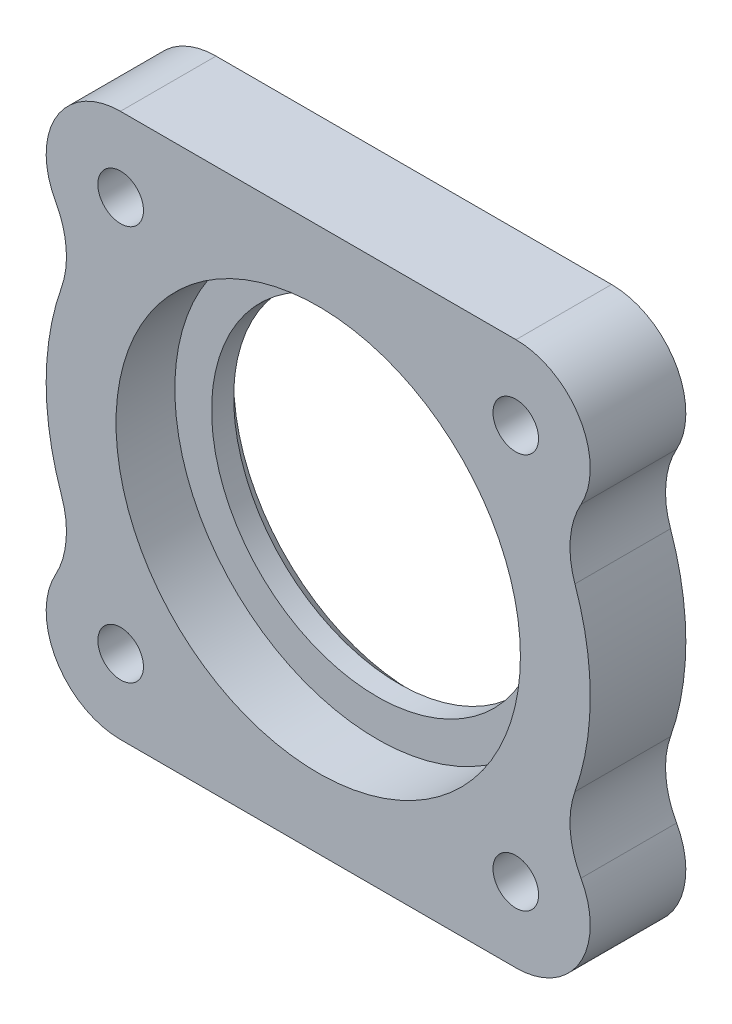
SolidWorks part; units mm, degrees
material "AL-1#"
ref_plane "前视基准面" through (0, 0, 0) normal (0, 0, 1) x (1, 0, 0)
ref_plane "上视基准面" through (0, 0, 0) normal (0, 1, 0) x (1, 0, 0)
ref_plane "右视基准面" through (0, 0, 0) normal (1, 0, 0) x (0, 0, -1)
sketch "草图1" plane through (0, 0, 0) normal (0, 0, 1) x (1, 0, 0)
  line L1 (-26.9, 37) -> (26.9, 37)
  line L5 (-37, 0) -> (-37, 44.6365) construction
  line L6 (26.9, 37) -> (26.9, 26.9) construction
  line L7 (-1000, 0) -> (49000, 0) construction
  line L10 (-26.9, 37) -> (-26.9, 26.9) construction
  line L12 (-37, 0) -> (37, 0)
  line L13 (0, -37) -> (0, 37) construction
  line L14 (-26.9, -37) -> (-26.9, -26.9) construction
  line L15 (26.9, -37) -> (26.9, -26.9) construction
  line L16 (-26.9, -37) -> (26.9, -37)
  arc A0 (-34.9172, 12.239) -> (-34.9172, -12.239) centre (0, 0) ccw
  arc A4 (-35.7394, 22.0138) -> (-26.9, 37) centre (-26.9, 26.9) cw
  arc A5 (-34.9172, 12.239) -> (-35.7394, 22.0138) centre (-46.2416, 16.2084) ccw
  arc A6 (34.9172, 12.239) -> (35.7394, 22.0138) centre (46.2416, 16.2084) cw
  arc A7 (35.7394, 22.0138) -> (26.9, 37) centre (26.9, 26.9) ccw
  arc A8 (34.9172, 12.239) -> (34.9172, -12.239) centre (0, 0) cw
  arc A9 (35.7394, -22.0138) -> (26.9, -37) centre (26.9, -26.9) cw
  arc A10 (34.9172, -12.239) -> (35.7394, -22.0138) centre (46.2416, -16.2084) ccw
  arc A11 (-34.9172, -12.239) -> (-35.7394, -22.0138) centre (-46.2416, -16.2084) cw
  arc A12 (-35.7394, -22.0138) -> (-26.9, -37) centre (-26.9, -26.9) ccw
  dimension "D2" = 10.1
  dimension "D5" = 24
extrude "凸台-拉伸1" add sketch "草图1" along normal blind 13 contours A11 A12 L16 A9 A10 A8 L12 A0 | A8 A6 A7 L1 A4 A5 A0 L12
sketch "草图2" plane through (0, 0, 13) normal (0, 0, 1) x (1, 0, 0)
  line L1 (-26.8701, 26.8701) -> (26.8701, 26.8701) construction
  line L2 (-26.8701, 26.8701) -> (-26.8701, -26.8701) construction
  line L3 (-26.8701, -26.8701) -> (26.8701, -26.8701) construction
  line L4 (26.8701, 26.8701) -> (26.8701, -26.8701) construction
  line L5 (-26.8701, 26.8701) -> (26.8701, -26.8701) construction
  line L6 (-26.8701, -26.8701) -> (26.8701, 26.8701) construction
  circle A0 centre (0, 0) radius 38 construction
  dimension "D1" = 76
hole_wizard "Ø6.2 (6.2) 直径孔1" positions "3D草图1" profile "草图3" hole size "Ø6.2" standard "GB" end condition up to next
sketch3d "3D草图1"
  point P0 (-26.8701, 26.8701, 13)
  point P3 (26.8701, 26.8701, 13)
  point P6 (26.8701, -26.8701, 13)
  point P9 (-26.8701, -26.8701, 13)
sketch "草图3" plane through (-26.8701, 26.8701, 13) normal (1, 0, 0) x (0, -1, 0)
  line L0 (0, 0) -> (0, 13)
  line L1 (0, 13) -> (3.1, 13)
  line L2 (3.1, 13) -> (3.1, 0)
  line L5 (3.1, 0) -> (0, 0)
  line L11 (0, -6.35) -> (0, 107.95) construction
  dimension "通孔孔直径" = 6.2
  dimension "通孔孔深度" = 13
sketch "草图4" plane through (0, 0, 13) normal (0, 0, 1) x (1, 0, 0)
  circle A0 centre (0, 0) radius 27.5
  dimension "D1" = 55
extrude "切除-拉伸1" cut sketch "草图4" against normal blind 8
sketch "草图5" plane through (0, 0, 5) normal (0, 0, 1) x (1, 0, 0)
  circle A0 centre (0, 0) radius 22.5
  dimension "D1" = 45
extrude "切除-拉伸2" cut sketch "草图5" against normal up to next
chamfer "倒角1" distance 2 angle 45 1 edges at (22.5, 0, 0)
